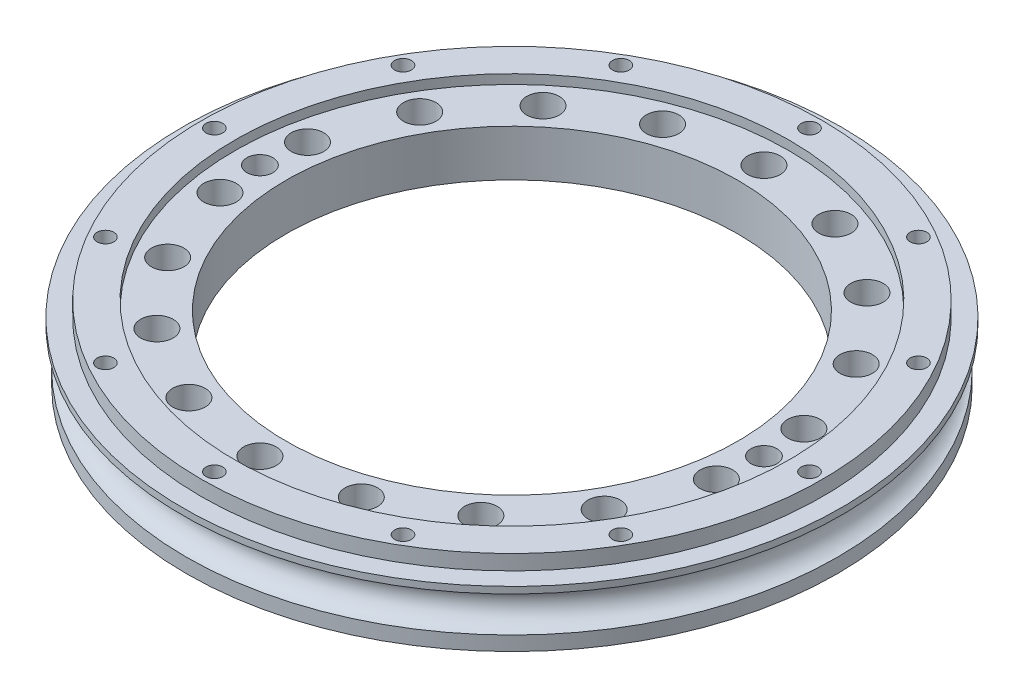
from build123d import *

# Parameters (mm, degrees)
CIRPATTERN1_COUNT            = 12
F_0_17_0_17_DIAMETER_HOLE1_D = 17.5
CIRPATTERN2_COUNT            = 18
M16_TAPPED_HOLE1_D           = 14
M16_TAPPED_HOLE1_DEPTH       = 35
M16_TAPPED_HOLE1_TIP         = 4.206024333


with BuildPart() as part:
    # Sketch1 → Revolve1 (revolve)
    with BuildSketch(Plane.XY, mode=Mode.PRIVATE) as revolve1_sk:
        with BuildLine():
            Line((-157, 0), (-175, 0))
            Line((-175, 0), (-175, 7.708741574))
            ThreePointArc((-175, 7.708741574), (-166.158424343, 19.100823753), (-177.2, 28.376415566))
            Line((-177.2, 28.376415566), (-177.2, 31.9))
            Line((-177.2, 31.9), (-167, 31.9))
            Line((-167, 31.9), (-167, 40))
            Line((-167, 40), (-149, 40))
            Line((-149, 40), (-149, 35))
            Line((-149, 35), (-121.5, 35))
            Line((-121.5, 35), (-121.5, 10))
            Line((-121.5, 10), (-157, 10))
            Line((-157, 10), (-157, 0))
        make_face()
    revolve(revolve1_sk.sketch.rotate(Axis((0, 22.704798349, 0), (0, 1, 0)), 270), axis=Axis((0, 22.704798349, 0), (0, 1, 0)))

    # Sketch2 → M10x1.0 Tapped Hole1 (revolve, cut)
    with BuildSketch(Plane(origin=(-160, 40, 0), x_dir=(0, 0, 1), z_dir=(1, 0, 0))):
        Polygon((0, 0), (0, 23.703872786), (4.5, 21), (4.5, 0), align=None)
    m10x1_0_tapped_hole1 = revolve(axis=Axis((-160, 46.35, 0), (0, -1, 0)), mode=Mode.SUBTRACT)

    # CirPattern1: M10x1.0 Tapped Hole1 ×12 about axis
    cirpattern1_axis = Axis((0, 0, 0), (0, 1, 0))
    for i in range(1, CIRPATTERN1_COUNT):
        add(m10x1_0_tapped_hole1.rotate(cirpattern1_axis, i * 360 / CIRPATTERN1_COUNT), mode=Mode.SUBTRACT)

    # Ø0.17 (0.17) Diameter Hole1 (through all)
    with Locations(Plane(origin=(0, 35, 0), x_dir=(-1, 0, 0), z_dir=(0, 1, 0))):
        with Locations((0, -135.5)):
            f_0_17_0_17_diameter_hole1 = Hole(F_0_17_0_17_DIAMETER_HOLE1_D / 2)

    # CirPattern2: Ø0.17 (0.17) Diameter Hole1 ×18 about axis
    cirpattern2_axis = Axis((0, 0, 0), (0, 1, 0))
    for i in range(1, CIRPATTERN2_COUNT):
        add(f_0_17_0_17_diameter_hole1.rotate(cirpattern2_axis, i * 360 / CIRPATTERN2_COUNT), mode=Mode.SUBTRACT)

    # M16 Tapped Hole1
    with Locations(Plane(origin=(0, 35, 0), x_dir=(-1, 0, 0), z_dir=(0, 1, 0))):
        with Locations((135.5, 0), (-135.5, 0)):
            Hole(M16_TAPPED_HOLE1_D / 2, depth=M16_TAPPED_HOLE1_DEPTH)
            with Locations((0, 0, -(M16_TAPPED_HOLE1_DEPTH + M16_TAPPED_HOLE1_TIP / 2))):  # 118° drill point
                Cone(0, M16_TAPPED_HOLE1_D / 2, M16_TAPPED_HOLE1_TIP, mode=Mode.SUBTRACT)


solid = part.part
